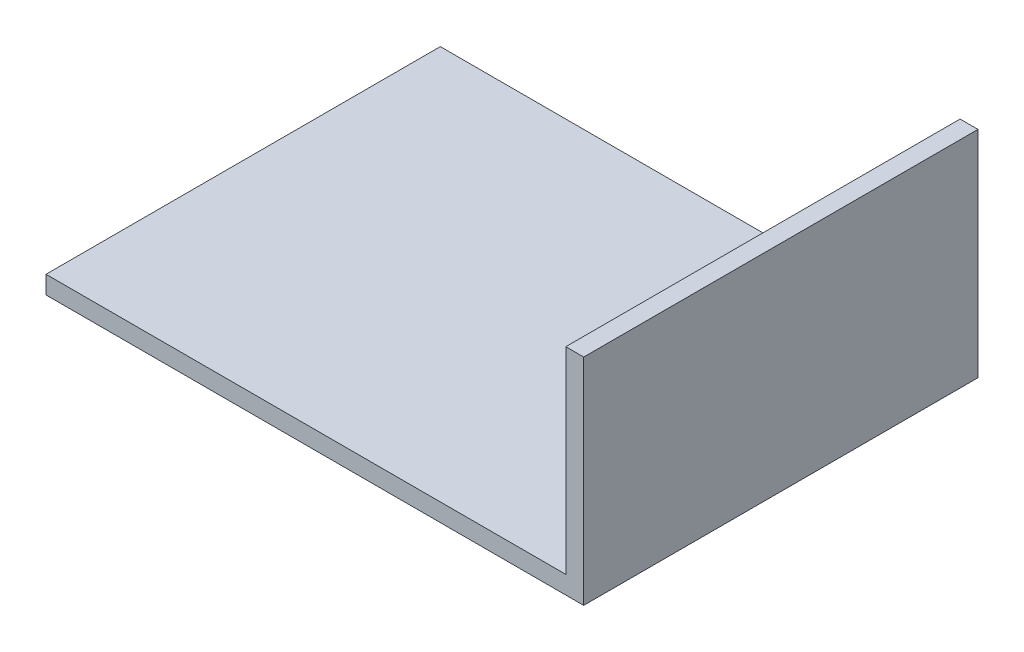
SolidWorks part; units mm, degrees
ref_plane "前视基准面" through (0, 0, 0) normal (0, 0, 1) x (1, 0, 0)
ref_plane "上视基准面" through (0, 0, 0) normal (0, 1, 0) x (1, 0, 0)
ref_plane "右视基准面" through (0, 0, 0) normal (1, 0, 0) x (0, 0, -1)
sketch "草图1" plane through (0, 0, 0) normal (0, 0, 1) x (1, 0, 0)
  line L0 (0, 0) -> (0, -60)
  line L1 (0, -60) -> (-150, -60)
  line L2 (-5, 0) -> (-5, -55)
  line L3 (-5, -55) -> (-150, -55)
  line L4 (-5, 0) -> (0, 0)
  line L5 (-150, -60) -> (-150, -55)
  dimension "D1" = 5
extrude "凸台-拉伸1" add sketch "草图1" along normal blind 110
